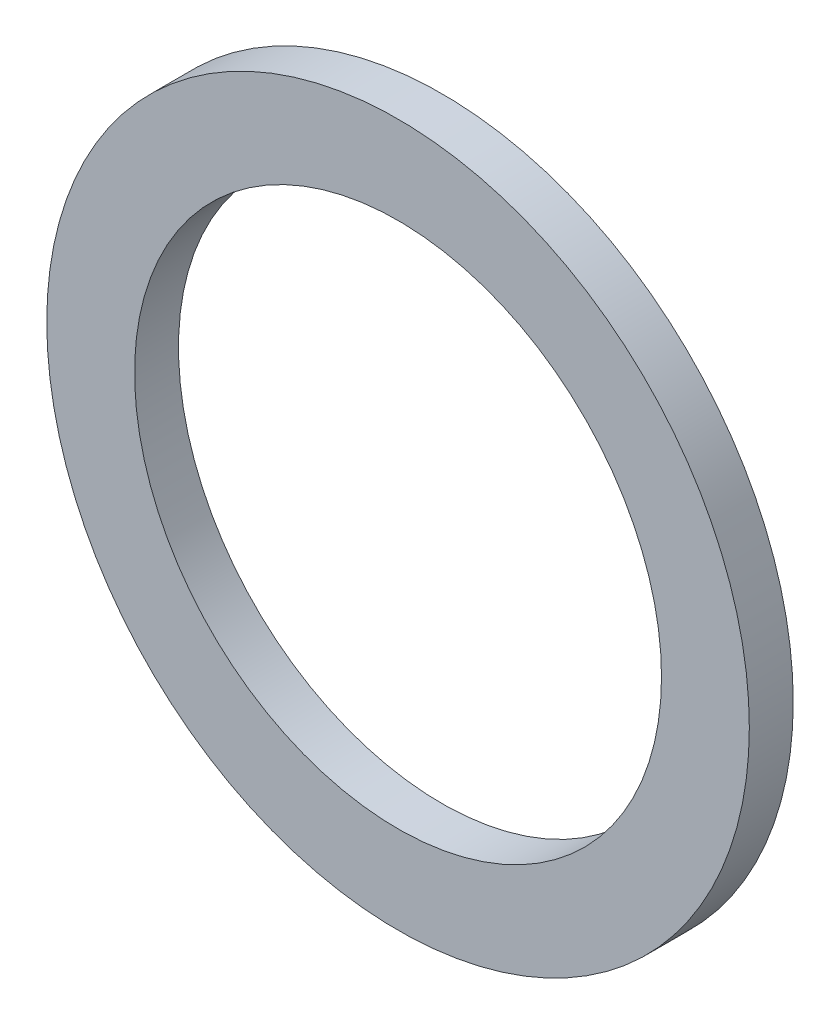
SolidWorks part; units mm, degrees
ref_plane "Front Plane" through (0, 0, 0) normal (0, 0, 1) x (1, 0, 0)
ref_plane "Top Plane" through (0, 0, 0) normal (0, 1, 0) x (1, 0, 0)
ref_plane "Right Plane" through (0, 0, 0) normal (1, 0, 0) x (0, 0, -1)
sketch "Sketch1" plane through (0, 0, 0) normal (0, 0, 1) x (1, 0, 0)
  circle A0 centre (0, 0) radius 8
  circle A1 centre (0, 0) radius 6
  dimension "D1" = 12
  dimension "D2" = 16
extrude "Boss-Extrude1" add sketch "Sketch1" along normal blind 1
